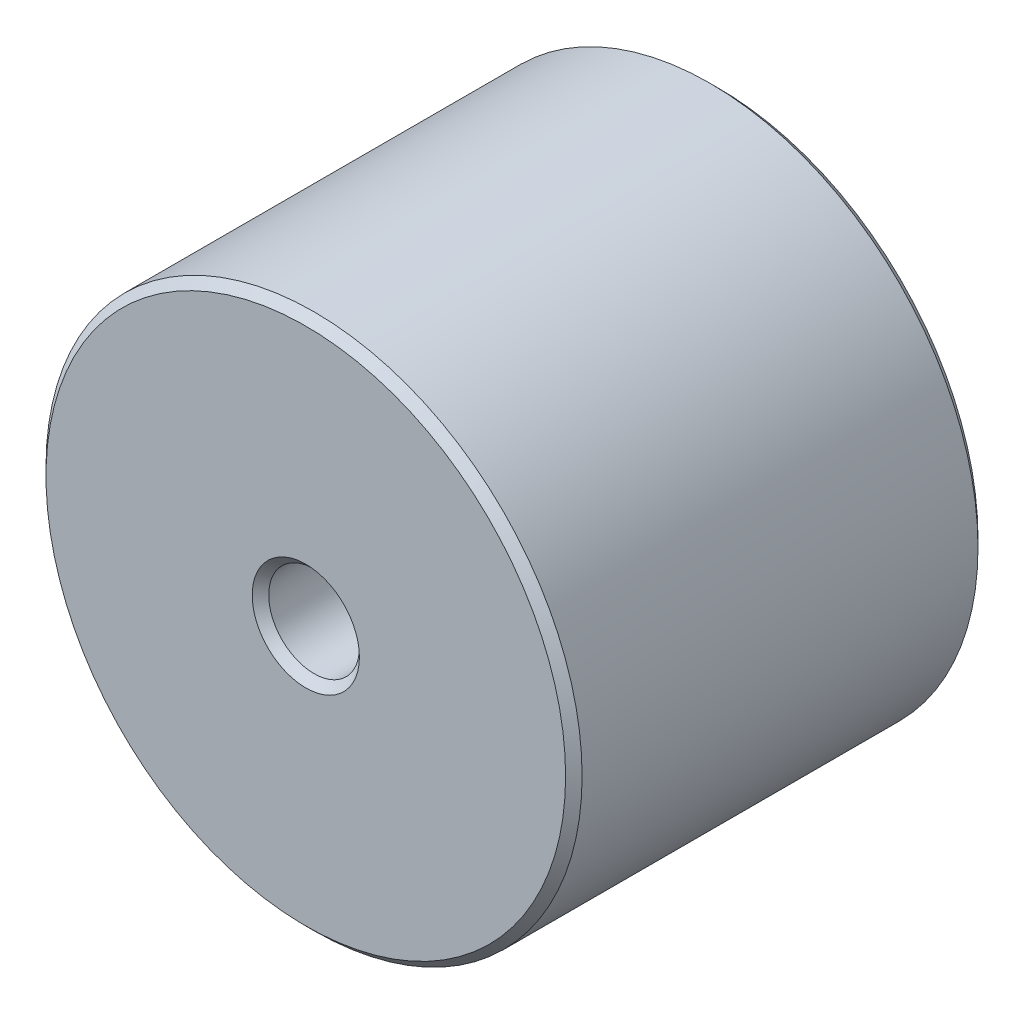
SolidWorks part; units mm, degrees
material "1023 碳钢板 (SS)"
ref_plane "前视基准面" through (0, 0, 0) normal (0, 0, 1) x (1, 0, 0)
ref_plane "上视基准面" through (0, 0, 0) normal (0, 1, 0) x (1, 0, 0)
ref_plane "右视基准面" through (0, 0, 0) normal (1, 0, 0) x (0, 0, -1)
sketch "草图1" plane through (0, 0, 0) normal (0, 0, 1) x (1, 0, 0)
  circle A0 centre (0, 0) radius 32.5
  circle A1 centre (0, 0) radius 5.5
  dimension "D1" = 65
  dimension "D2" = 11
extrude "凸台-拉伸1" add sketch "草图1" along normal blind 50
chamfer "倒角1" distance 1 angle 45 4 edges at (5.5, 0, 0) (32.5, 0, 0) (5.5, 0, 50) (32.5, 0, 50)
